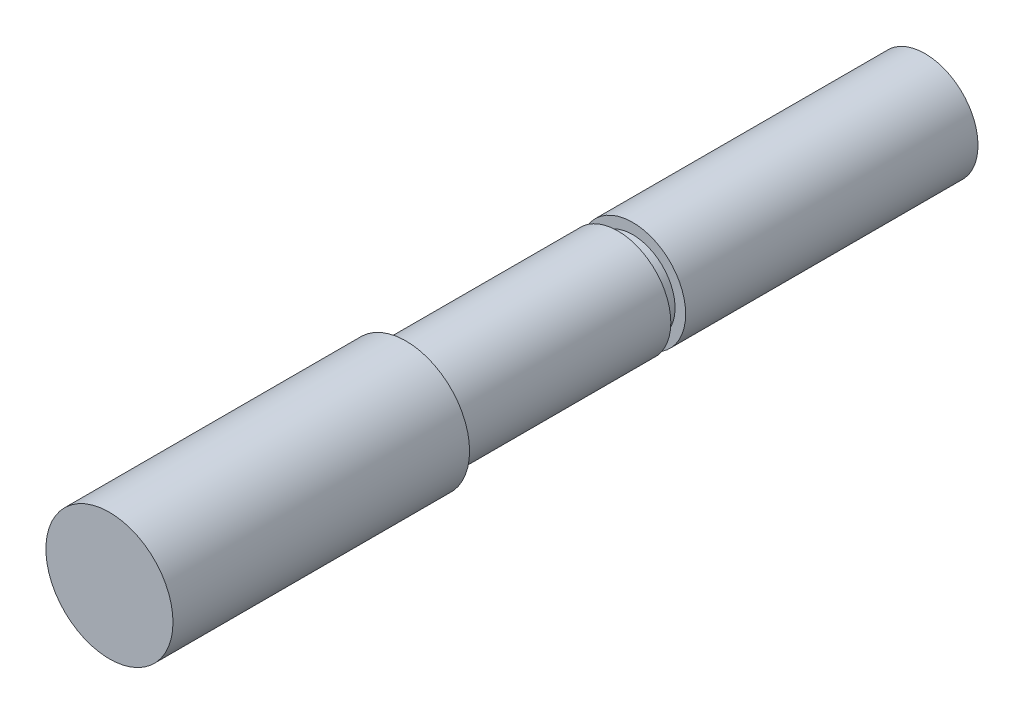
SolidWorks part; units mm, degrees
ref_plane "前视基准面" through (0, 0, 0) normal (0, 0, 1) x (1, 0, 0)
ref_plane "上视基准面" through (0, 0, 0) normal (0, 1, 0) x (1, 0, 0)
ref_plane "右视基准面" through (0, 0, 0) normal (1, 0, 0) x (0, 0, -1)
sketch "草图1" plane through (0, 0, 0) normal (0, 0, 1) x (1, 0, 0)
  circle A0 centre (0, 0) radius 3
  dimension "D1" = 6
extrude "凸台-拉伸1" add sketch "草图1" along normal blind 14
sketch "草图2" plane through (0, 0, 0) normal (0, 0, -1) x (-1, 0, 0)
  circle A0 centre (0, 0) radius 2.5
  dimension "D1" = 5
extrude "凸台-拉伸2" add sketch "草图2" along normal blind 24.5
sketch "草图3" plane through (0, 0, 0) normal (0, 1, 0) x (1, 0, 0)
  line L0 (0, 21.4746) -> (0, -2.9286) construction
  line L1 (2, 10.7) -> (3.9817, 10.7)
  line L2 (2, 10.7) -> (2, 10)
  line L3 (2, 10) -> (3.9817, 10)
  line L4 (3.9817, 10.7) -> (3.9817, 10)
  line L5 (2, 10.7) -> (3.9817, 10) construction
  line L6 (2, 10) -> (3.9817, 10.7) construction
  line L7 (3, 0) -> (-3, 0) construction
  point P0 (2.9909, 10.35)
  dimension "D1" = 2
  dimension "D2" = 0.7
  dimension "D3" = 10
revolve "切除-旋转1" cut sketch "草图3" angle 360 about L0
